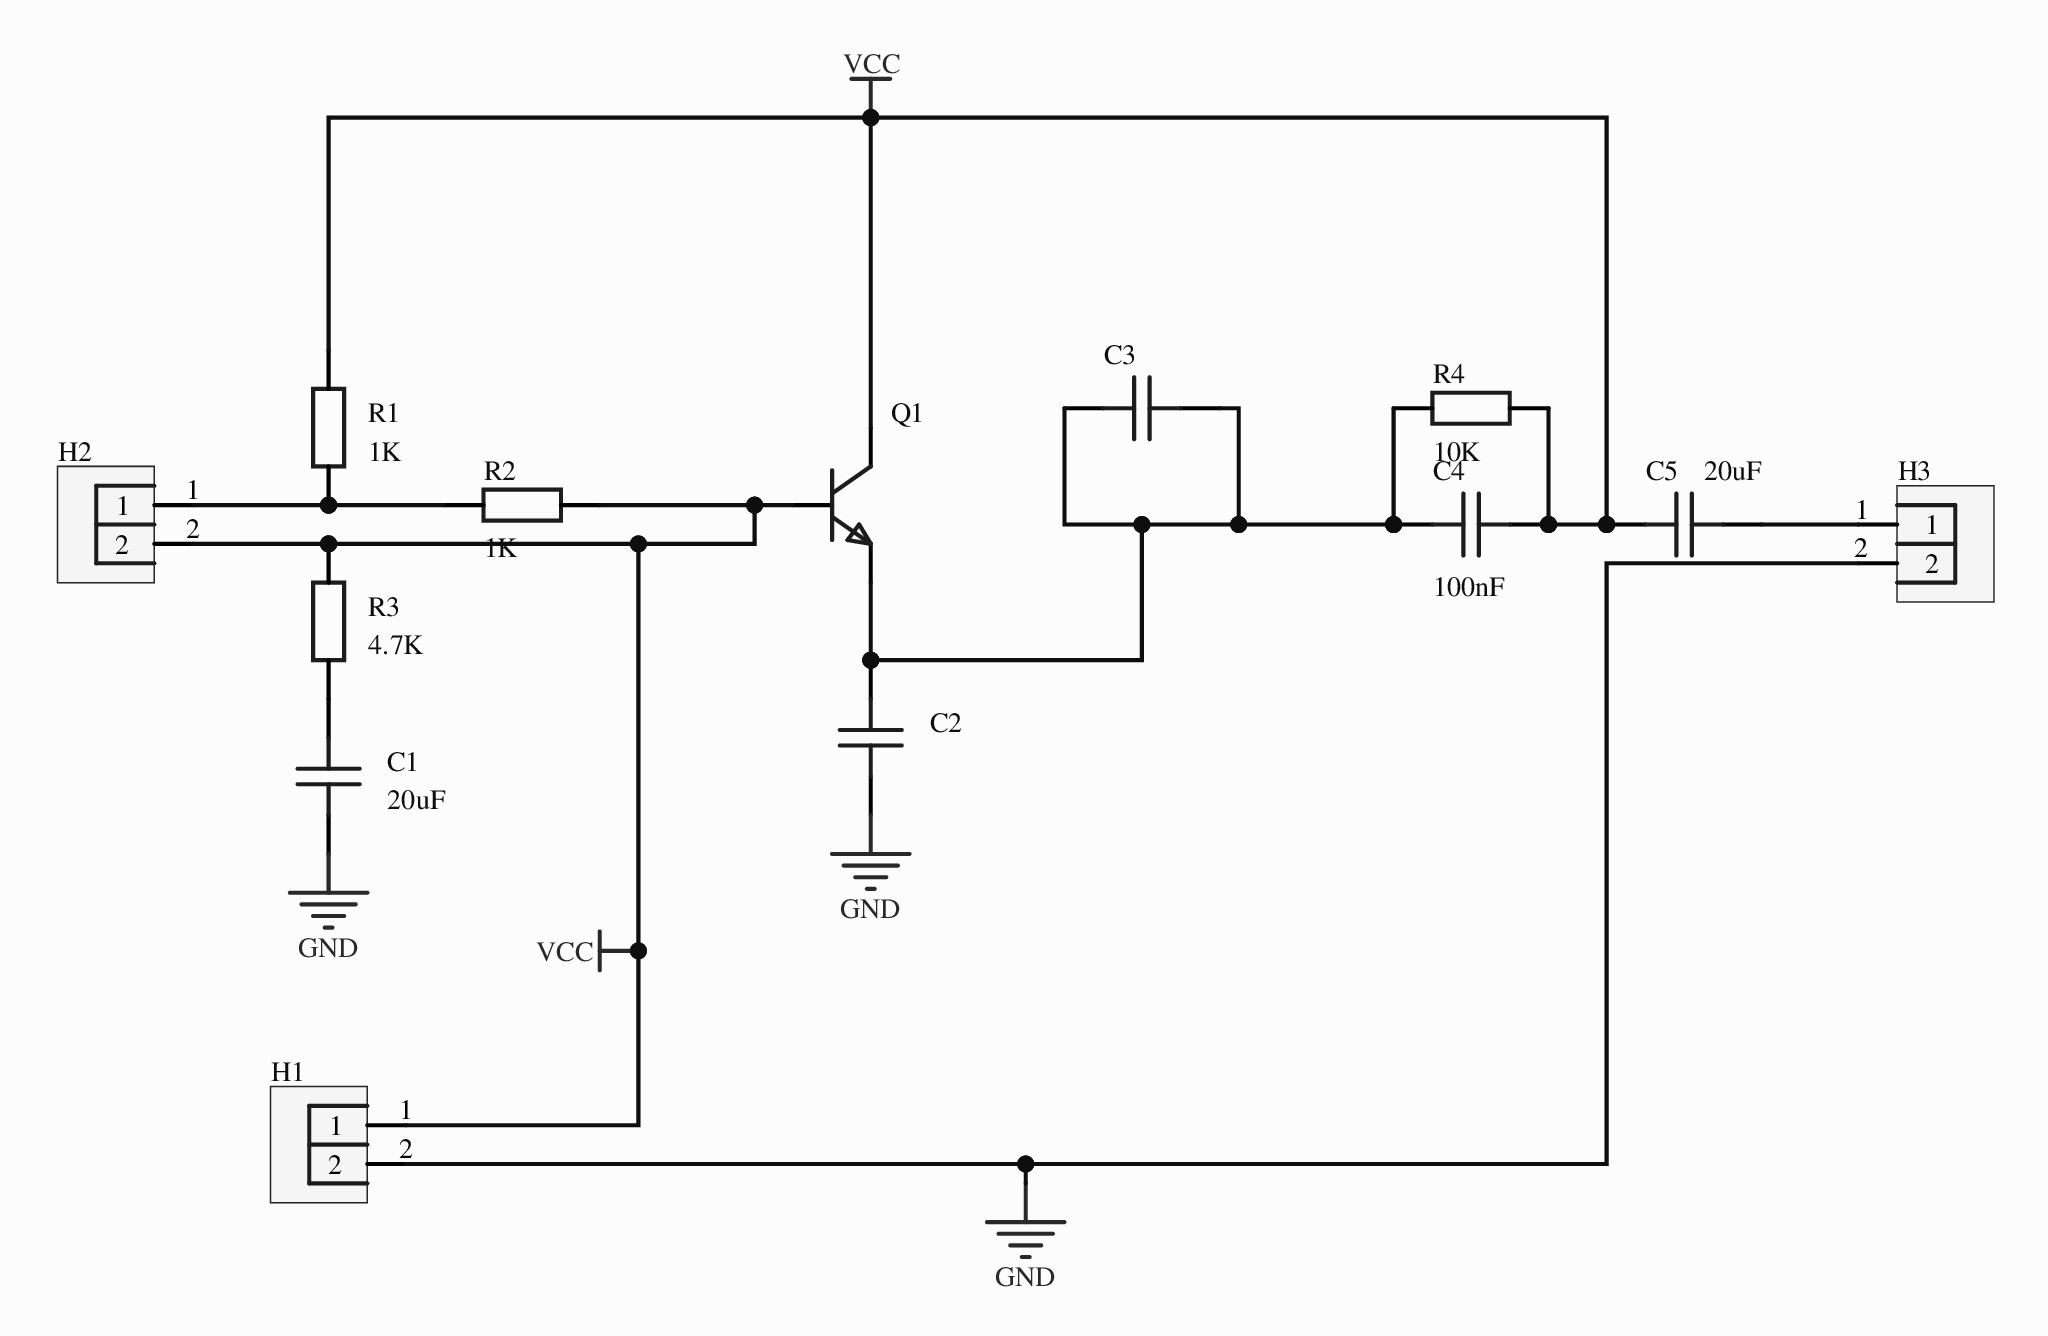
[diagram p0: MISC52148-3.schdoc]
# Altium project MISC52148-2.PrjPcb
1 sheet, 13 parts. Net scope: global (net labels, ports and power ports of the same name join across sheets).
Board file: MISC52148.pcbdoc

## Sheet MISC52148-3.schdoc
size 210 x 148 mm; Version: V1.0; @Project Name: MISC52148; @Update Date: 2026-10-07; @Create Date: 2026-10-07; @Board Name: MISC52148; @Create Time: 12:44:54; @Page Count: 1; @Page No: 1; @Schematic Name: MISC52148; @Update Time: 12:44:54; Size: A4

### Parts
C1  20uF  [C0603]
C2  100nF  [C0603]  (value not drawn)
C3  100nF  [C0603]  (value not drawn)
C4  100nF  [C0603]
C5  20uF  [C0603]
H1  (no value)  [HDR-TH_2P-P2.54-V-M-1]
H2  (no value)  [HDR-TH_2P-P2.54-V-M-1]
H3  (no value)  [HDR-TH_2P-P2.54-V-M-1]
Q1  (no value)  [S8050_SOT-23]
R1  1K  [R0603]
R2  1K  [R0603]
R3  4.7K  [R0603]
R4  10K  [R0603]

### Nets
GND: C1.1 C2.1 H1.2 H3.2
VCC: C4.2 C5.1 H1.1 H2.2 Q1.1 Q1.3 R1.2 R2.1 R3.2 R4.2
NetC1_2: C1.2 R3.1
NetC2_2: C2.2 C3.1 C3.2 C4.1 Q1.2 R4.1
NetC5_2: C5.2 H3.1
NetH2_1: H2.1 R1.1 R2.2

### Library data of the parts
C1-C5 = CAP_0603: Symbol: Capacitance; 3D Model: ac125912035d415993ca9572d50418b10819f05c4eef4c71ace90d822a990e87; 3D Model Transform: 62.992,31.496,0,0,0,0,0,0,0; ConvertToPcb: yes; ModelName: C0603_L1.6-W0.8-H0.8; Device: CAP_0603; Supplier Footprint: 0603; FootprintName: C0603; AddInBom: yes
  C1 C5: Value: 20uF
  C2-C4: Value: 100nF
H1-H3 = HDR-M_2.54_1x2P: Symbol: 210S-1*2P L=11.6MMGold-plated black; 3D Model: 79b2e9f2d70a4d68a1b7098f27c6d4c50819f05c4eef4c71ace90d822a990e87; 3D Model Transform: 200,100,0,0,0,0,0,0,-118.11; ConvertToPcb: yes; ModelName: HDR-M-2.54_1x2; Device: HDR-M_2.54_1x2P; Supplier Part: C124375; Supplier Footprint: 插件; FootprintName: HDR-TH_2P-P2.54-V-M-1; AddInBom: yes
Q1 = S8050_SOT_NPN: Symbol: NPN; ConvertToPcb: yes; ModelId: c62791f0466c4ae2a892c056b845b0ca0819f05c4eef4c71ace90d822a990e87; ModelName: SOT-23-3P_L2.9-W1.3-H1.0-LS2.4-P0.95; ModelTransform: 98.6,114.12,41.29,180,0,0,0,0,-3; Device: S8050_SOT_NPN; FootprintName: S8050_SOT-23; AddInBom: yes; Supplier Footprint: SOT-23
R1-R4 = Res_0603: Symbol: Resistor; 3D Model: fc143cca1e79419f9cd78b61e9279f080819f05c4eef4c71ace90d822a990e87; 3D Model Transform: 31.8897,63.7794,0,90,0,0,0,0,0; ConvertToPcb: yes; Device: Res_0603; Supplier Footprint: 0603; FootprintName: R0603; AddInBom: yes; ModelName: R0603
  R1 R2: Value: 1K
  R3: Value: 4.7K
  R4: Value: 10K